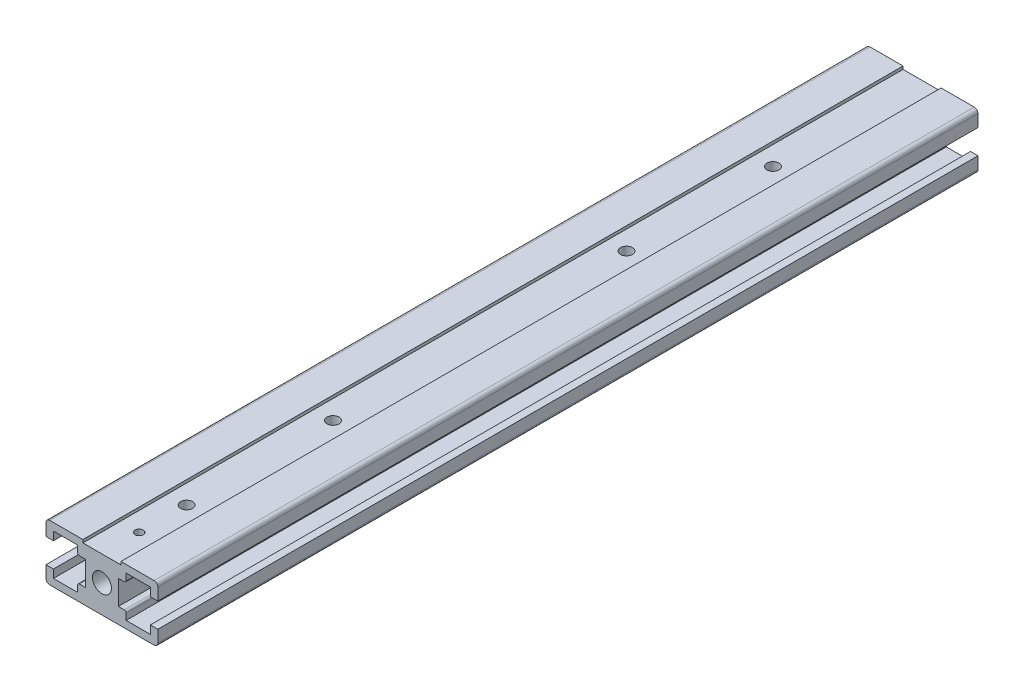
from build123d import *

# Parameters (mm, degrees)
SKETCH_1_W             = 30
SKETCH_1_H             = 15
EXTRUDE_1_DEPTH        = 220
FILLET_1_R             = 1
SKETCH_2_R             = 2.55
CUT_EXTRUDE_1_DEPTH    = 230
SKETCH_3_W             = 21.2
SKETCH_3_H             = 6.55
CUT_EXTRUDE_2_DEPTH    = 230
SKETCH_4_W             = 6.5
SKETCH_4_H             = 11
CUT_EXTRUDE_3_DEPTH    = 230
FILLET_2_R             = 0.5
SKETCH_5_R             = 1.6
CUT_EXTRUDE_4_DEPTH    = 10
PATTERN_LINEAR_1_COUNT = 2
PATTERN_LINEAR_1_PITCH = 118
SKETCH_6_R             = 1.1
CUT_EXTRUDE_5_DEPTH    = 222.020361153
SKETCH_7_W             = 10.2
SKETCH_7_H             = 220
CUT_EXTRUDE_6_DEPTH    = 0.8


with BuildPart() as part:
    # 草图1 → 凸台-拉伸1 (new body)
    with BuildSketch(Plane.XY):
        Rectangle(SKETCH_1_W, SKETCH_1_H)
    extrude(amount=EXTRUDE_1_DEPTH)

    # 圆角1
    fillet_1_edges = [part.edges().sort_by_distance(p)[0] for p in [
        (15, -7.5, 110),
        (-15, -7.5, 110),
        (-15, 7.5, 110),
        (15, 7.5, 110),
    ]]
    fillet(fillet_1_edges, radius=FILLET_1_R)

    # 草图2 → 切除-拉伸1 (cut)
    with BuildSketch(Plane.XY.offset(220)):
        Circle(SKETCH_2_R)
    extrude(amount=-CUT_EXTRUDE_1_DEPTH, mode=Mode.SUBTRACT)

    # 草图3 → 切除-拉伸2 (cut)
    with BuildSketch(Plane.XY.offset(220)):
        with Locations((-15, -0.025)):
            Rectangle(SKETCH_3_W, SKETCH_3_H)
    cut_extrude_2 = extrude(amount=-CUT_EXTRUDE_2_DEPTH, mode=Mode.SUBTRACT)

    # 镜向1: 切除-拉伸2 across plane
    add(cut_extrude_2.mirror(Plane(origin=(0, 0, 0), x_dir=(0, 0, 1), z_dir=(1, 0, 0))), mode=Mode.SUBTRACT)

    # 草图4 → 切除-拉伸3 (cut)
    with BuildSketch(Plane.XY.offset(220)):
        with Locations((-9.75, 0)):
            Rectangle(SKETCH_4_W, SKETCH_4_H)
    cut_extrude_3 = extrude(amount=-CUT_EXTRUDE_3_DEPTH, mode=Mode.SUBTRACT)

    # 镜向2: 切除-拉伸3 across plane
    add(cut_extrude_3.mirror(Plane(origin=(0, 0, 0), x_dir=(0, 0, 1), z_dir=(1, 0, 0))), mode=Mode.SUBTRACT)

    # 圆角2
    fillet_2_edges = [part.edges().sort_by_distance(p)[0] for p in [
        (6.5, -3.3, 110),
        (6.5, 3.25, 110),
        (-6.5, 3.25, 110),
        (-6.5, -3.3, 110),
    ]]
    fillet(fillet_2_edges, radius=FILLET_2_R)

    # 草图5 → 切除-拉伸4 (cut)
    with BuildSketch(Plane(origin=(0, 7.5, 0), x_dir=(1, 0, 0), z_dir=(0, 1, 0))):
        with Locations(Location((0, -40, 0), (0, 0, 270))):
            Circle(SKETCH_5_R)
        with Locations(Location((0, -79.285714286, 0), (0, 0, 270))):
            Circle(SKETCH_5_R)
    cut_extrude_4 = extrude(amount=-CUT_EXTRUDE_4_DEPTH, mode=Mode.SUBTRACT)

    # 阵列(线性)1: 切除-拉伸4 ×2
    with Locations(*[(0, 0, i * PATTERN_LINEAR_1_PITCH) for i in range(1, PATTERN_LINEAR_1_COUNT)]):
        add(cut_extrude_4, mode=Mode.SUBTRACT)

    # 草图6 → 切除-拉伸5 (cut, through all)
    with BuildSketch(Plane(origin=(0, 7.5, 0), x_dir=(1, 0, 0), z_dir=(0, 1, 0))):
        with Locations(Location((0, -210, 0), (0, 0, 270))):
            Circle(SKETCH_6_R)
    extrude(amount=-CUT_EXTRUDE_5_DEPTH, mode=Mode.SUBTRACT)

    # 草图7 → 切除-拉伸6 (cut)
    with BuildSketch(Plane(origin=(0, 7.5, 0), x_dir=(1, 0, 0), z_dir=(0, 1, 0))):
        with Locations((0, -110)):
            Rectangle(SKETCH_7_W, SKETCH_7_H)
    extrude(amount=-CUT_EXTRUDE_6_DEPTH, mode=Mode.SUBTRACT)


solid = part.part
